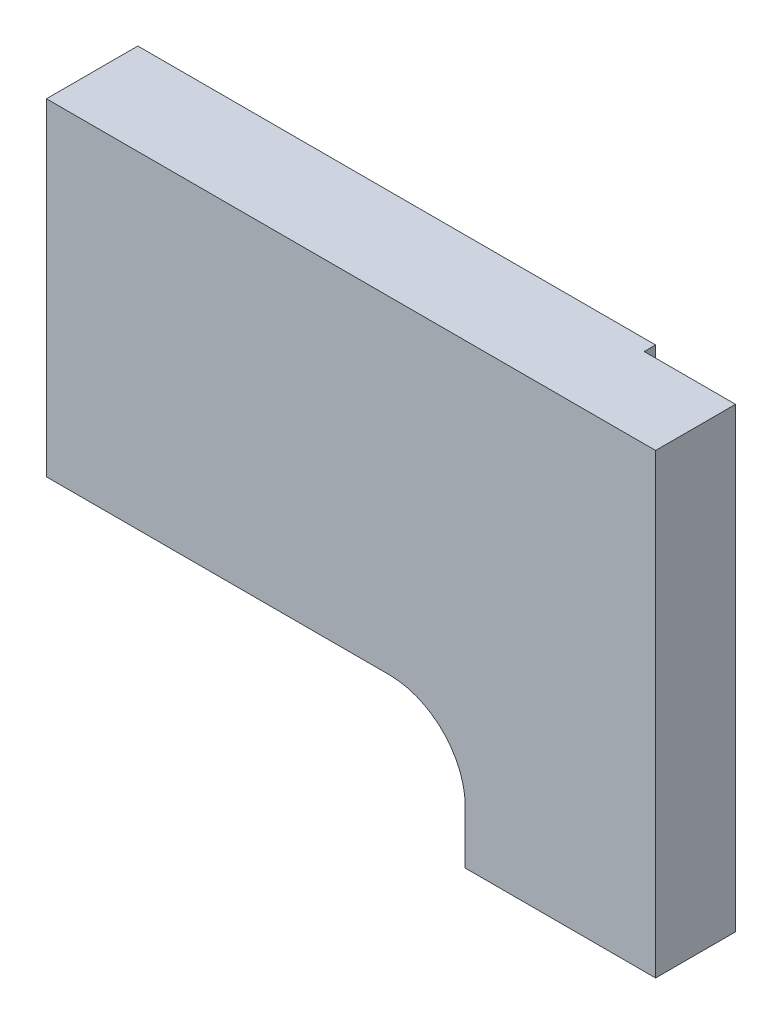
from build123d import *

# Parameters (mm, degrees)
SKETCH_1_W          = 80
SKETCH_1_H          = 60
EXTRUDE_1_DEPTH     = 6
SKETCH_2_W          = 12
SKETCH_2_H          = 60
CUT_EXTRUDE_1_DEPTH = 1.5
CUT_EXTRUDE_2_REACH = 53.42
SKETCH_3_W          = 55
SKETCH_3_H          = 17
FILLET_1_R          = 10


with BuildPart() as part:
    # 草图1 → 凸台-拉伸1 (new, symmetric)
    with BuildSketch(Plane.XY):
        Rectangle(SKETCH_1_W, SKETCH_1_H)
    extrude(amount=EXTRUDE_1_DEPTH, both=True)

    # 草图2 → 切除-拉伸1 (cut)
    with BuildSketch(Plane.XY.offset(-6)):
        with Locations((34, 0)):
            Rectangle(SKETCH_2_W, SKETCH_2_H)
    extrude(amount=CUT_EXTRUDE_1_DEPTH, mode=Mode.SUBTRACT)

    # 草图3 → 切除-拉伸2 (cut, up to next)
    with BuildSketch(Plane(origin=(0, 0, -6), x_dir=(-1, 0, 0), z_dir=(0, 0, -1)), mode=Mode.PRIVATE) as cut_extrude_2_sk1:
        with Locations((12.5, -21.5)):
            Rectangle(SKETCH_3_W, SKETCH_3_H)
    cut_extrude_2_tool1 = extrude(cut_extrude_2_sk1.sketch, amount=-CUT_EXTRUDE_2_REACH, mode=Mode.PRIVATE) & part.part
    add(cut_extrude_2_tool1.solids().sort_by_distance((-12.5, -21.5, -6))[0], mode=Mode.SUBTRACT)

    # 圆角1
    fillet_1_edges = [part.edges().sort_by_distance(p)[0] for p in [
        (15, -13, 0),
    ]]
    fillet(fillet_1_edges, radius=FILLET_1_R)


solid = part.part
